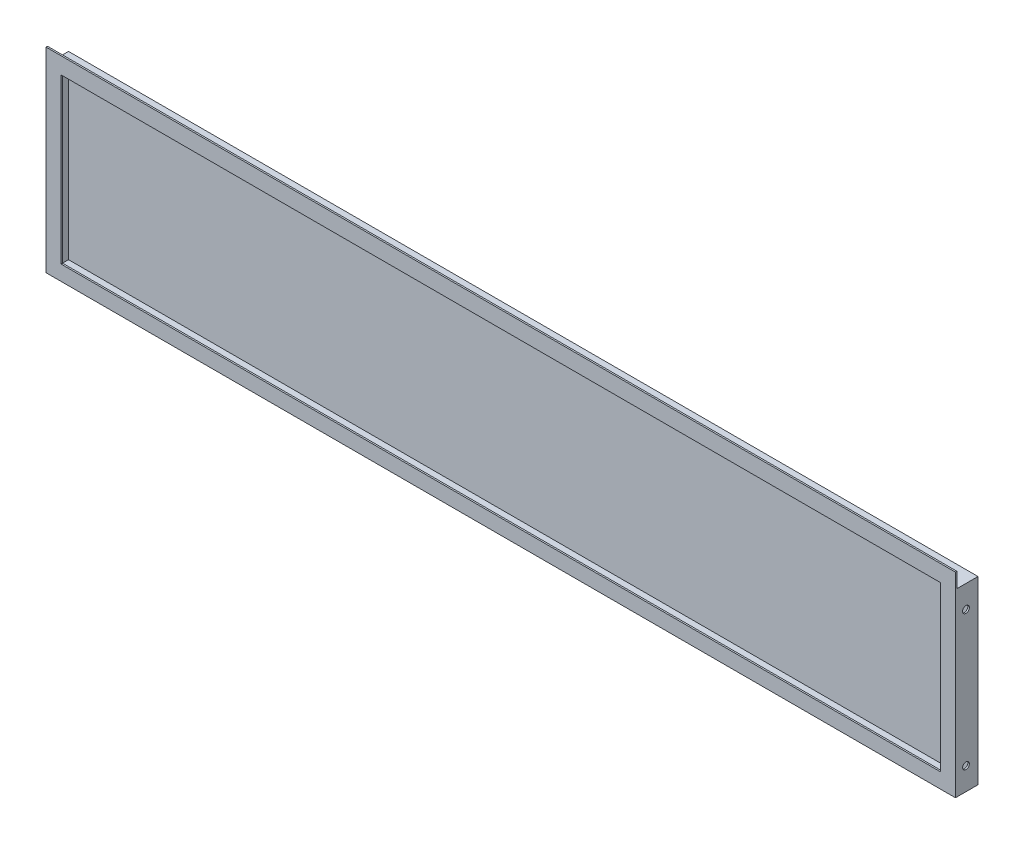
SolidWorks part; units mm, degrees
ref_plane "前视基准面" through (0, 0, 0) normal (0, 0, 1) x (1, 0, 0)
ref_plane "上视基准面" through (0, 0, 0) normal (0, 1, 0) x (1, 0, 0)
ref_plane "右视基准面" through (0, 0, 0) normal (1, 0, 0) x (0, 0, -1)
sketch "草图1" plane through (0, 0, 0) normal (0, 0, 1) x (1, 0, 0)
  line L1 (0, 0) -> (1210, 0)
  line L2 (0, 0) -> (0, 240)
  line L3 (0, 240) -> (1210, 240)
  line L4 (1210, 0) -> (1210, 240)
  dimension "D1" = 240
  dimension "D2" = 1210
extrude "凸台-拉伸1" add sketch "草图1" along normal blind 30
shell "抽壳1" thickness 2
sketch "草图2" plane through (0, 0, 30) normal (0, 0, 1) x (1, 0, 0)
  line L0 (1208, 238) -> (2, 238) construction
  line L1 (0, 260) -> (1210, 260)
  line L2 (0, 260) -> (0, 0)
  line L3 (0, 0) -> (1210, 0)
  line L4 (1210, 260) -> (1210, 0)
  line L5 (0, 240) -> (0, 0) construction
  line L6 (1210, 240) -> (0, 240) construction
  line L7 (1208, 238) -> (2, 238) construction
  line L8 (20, 20) -> (1190, 20)
  line L9 (20, 20) -> (20, 238)
  line L10 (20, 238) -> (1190, 238)
  line L11 (1190, 20) -> (1190, 238)
  dimension "D1" = 20
  dimension "D2" = 20
  dimension "D3" = 20
  dimension "D4" = 20
extrude "凸台-拉伸2" add sketch "草图2" against normal blind 2
sketch "草图3" plane through (2, 0, 0) normal (1, 0, 0) x (0, 0, -1)
  line L0 (-16, 2) -> (-16, 255.9498) construction
  line L3 (-28, 2) -> (-2, 2) construction
  line L4 (-30, 260) -> (-30, 0) construction
  line L5 (-30, 0) -> (0, 0) construction
  line L6 (-28, 240) -> (0, 240) construction
  circle A0 centre (-16, 30) radius 4.5
  circle A1 centre (-16, 210) radius 4.5
  dimension "D2" = 9
  dimension "D3" = 9
  dimension "D4" = 30
  dimension "D5" = 30
  dimension "D1" = 14
extrude "切除-拉伸1" cut sketch "草图3" along normal blind 1316 and the other way blind 198
sketch "草图4" plane through (0, 2, 0) normal (0, 1, 0) x (1, 0, 0)
  line L0 (-38.2949, -16) -> (1398.2949, -16) construction
  line L1 (1210, -30) -> (0, -30) construction
  line L2 (1210, -28) -> (1210, 0) construction
  line L3 (0, -28) -> (0, 0) construction
  line L4 (1210, -30) -> (1210, 0) construction
  circle A0 centre (30, -16) radius 4.5
  circle A1 centre (1180, -16) radius 4.5
  circle A2 centre (680, -16) radius 4.5
  circle A3 centre (320, -16) radius 4.5
  circle A4 centre (740, -16) radius 4.5
  dimension "D2" = 9
  dimension "D3" = 9
  dimension "D4" = 30
  dimension "D5" = 30
  dimension "D6" = 9
  dimension "D7" = 9
  dimension "D8" = 530
  dimension "D10" = 9
  dimension "D11" = 470
  dimension "D1" = 14
  dimension "D9" = 890
extrude "切除-拉伸2" cut sketch "草图4" against normal blind 45
